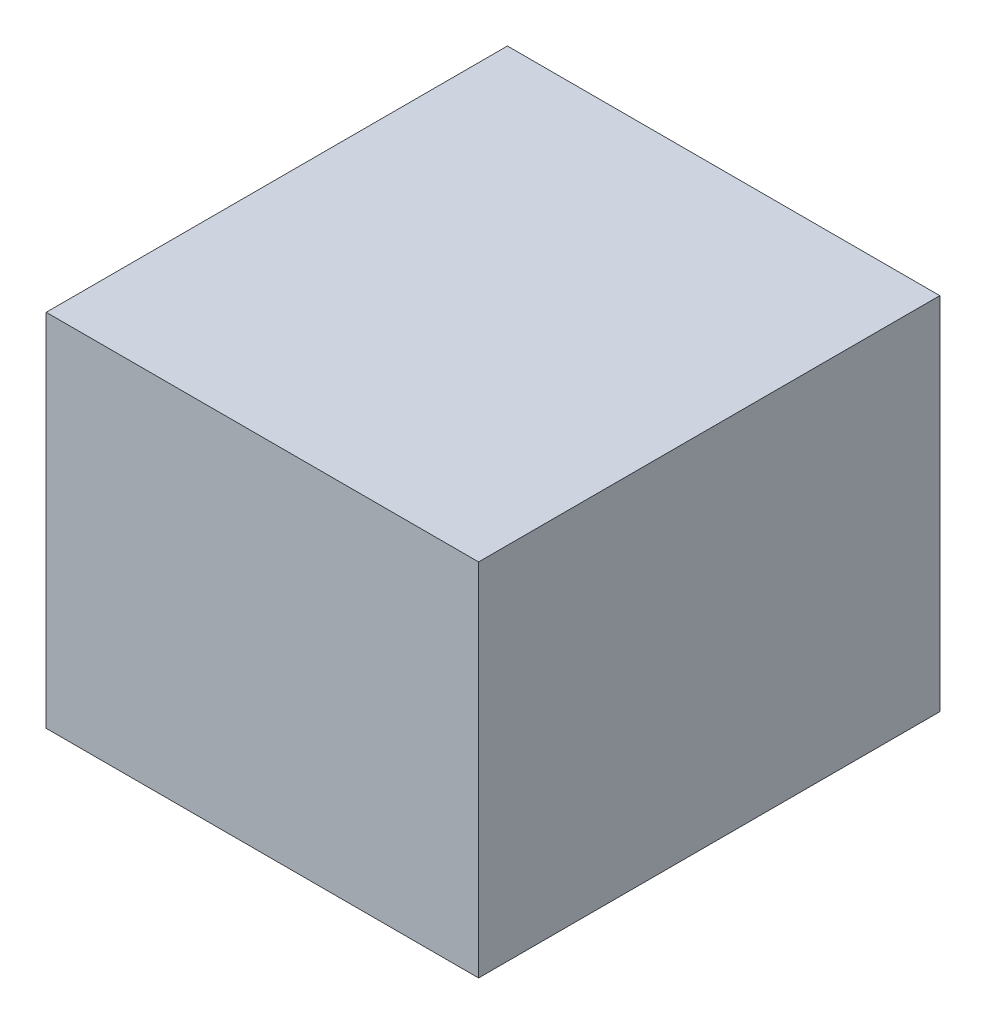
from build123d import *

# Parameters (mm, degrees)
SKETCH1_W           = 300
SKETCH1_H           = 320
BOSS_EXTRUDE1_DEPTH = 250


with BuildPart() as part:
    # Sketch1 → Boss-Extrude1 (new body)
    with BuildSketch(Plane(origin=(0, 0, 0), x_dir=(1, 0, 0), z_dir=(0, 1, 0))):
        Rectangle(SKETCH1_W, SKETCH1_H)
    extrude(amount=BOSS_EXTRUDE1_DEPTH)


solid = part.part
